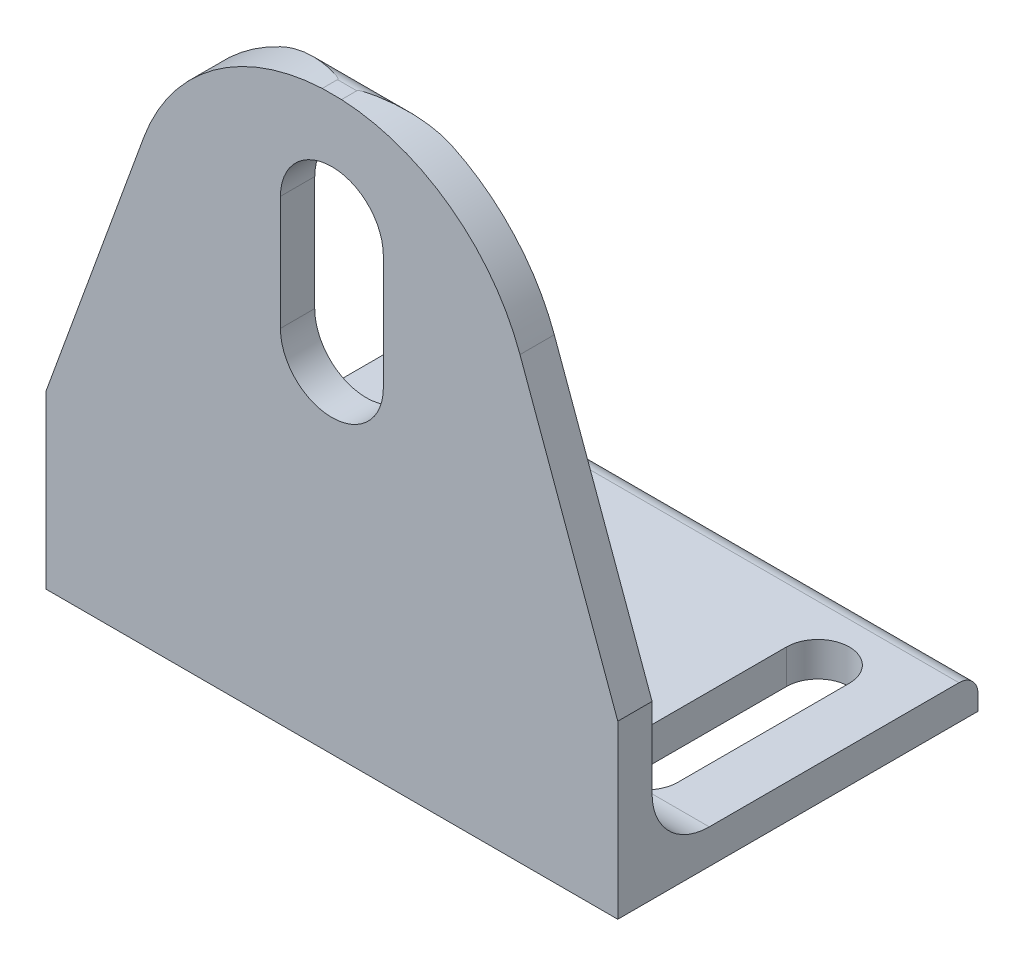
SolidWorks part; units mm, degrees
material "普通碳钢"
ref_plane "Front Plane" through (0, 0, 0) normal (0, 0, 1) x (1, 0, 0)
ref_plane "Top Plane" through (0, 0, 0) normal (0, 1, 0) x (1, 0, 0)
ref_plane "Right Plane" through (0, 0, 0) normal (1, 0, 0) x (0, 0, -1)
sketch3d "3DSketch1"
  line L0 (0, 0, 0) -> (100, 0, 0)
  dimension "D1" = 100
other "Hot-rolled unequal angle gb∕t706-2008 100 X 63 X 6(1)"
ref_plane "Plane1" through (0, 0, 0) normal (1, 0, 0) x (0, 0, -1)
sketch "Sketch1" plane through (0, 0, 0) normal (1, 0, 0) x (0, 0, -1)
  line L0 (0, 0) -> (0, 100)
  line L1 (0, 50) -> (6, 50) construction
  line L2 (6, 96.6667) -> (6, 16)
  line L3 (16, 6) -> (59.6667, 6)
  line L4 (31.5, 6) -> (31.5, 0) construction
  line L5 (63, 0) -> (0, 0)
  line L6 (0, 100) -> (2.6667, 100)
  line L7 (63, 0) -> (63, 2.6667)
  arc A0 (63, 2.6667) -> (59.6667, 6) centre (59.6667, 2.6667) ccw
  arc A1 (2.6667, 100) -> (6, 96.6667) centre (2.6667, 96.6667) cw
  arc A2 (16, 6) -> (6, 16) centre (16, 16) cw
  point P10 (31.5, 0)
  point P14 (0, 50)
  point P15 (6, 50)
  point P16 (31.5, 6)
  point P21 (0, 0)
sketch "Sketch3" plane through (0, 0, 0) normal (0, 0, 1) x (1, 0, 0)
  line L0 (50, 115) -> (50, 0) construction
  line L2 (0, 0) -> (100, 0) construction
  line L3 (50, 80) -> (50, 60) construction
  line L4 (59, 80) -> (59, 60)
  line L5 (41, 80) -> (41, 60)
  line L6 (0, 30) -> (17.101, 76.9846)
  line L7 (0, 100) -> (0, 0) construction
  line L8 (0, 30) -> (0, 0)
  line L9 (0, 0) -> (100, 0)
  line L10 (100, 0) -> (100, 30)
  line L11 (100, 100) -> (100, 0) construction
  line L12 (100, 30) -> (82.899, 76.9846)
  arc A0 (59, 80) -> (41, 80) centre (50, 80) ccw
  arc A1 (41, 60) -> (59, 60) centre (50, 60) ccw
  arc A2 (17.101, 76.9846) -> (82.899, 76.9846) centre (50, 65.0408) cw
  point P8 (50, 70)
  dimension "D6" = 160
  dimension "D8" = 50
  dimension "D9" = 35
  dimension "D1" = 18
  dimension "D2" = 20
  dimension "D3" = 60
  dimension "D4" = 30
  dimension "D5" = 30
  dimension "D7" = 160
extrude "Cut-Extrude1" cut sketch "Sketch3" against normal blind 10 flip side to cut
sketch "Sketch4" plane through (0, 0, 0) normal (0, -1, 0) x (1, 0, 0)
  line L0 (50, 0) -> (50, -67.1057) construction
  line L1 (0, 0) -> (100, 0) construction
  line L3 (15, -20) -> (15, -50) construction
  line L4 (20.5, -20) -> (20.5, -50)
  line L5 (9.5, -20) -> (9.5, -50)
  line L6 (85, -20) -> (85, -50) construction
  line L7 (79.5, -20) -> (79.5, -50)
  line L8 (90.5, -20) -> (90.5, -50)
  line L9 (100, 0) -> (0, 0) construction
  arc A0 (20.5, -20) -> (9.5, -20) centre (15, -20) ccw
  arc A1 (9.5, -50) -> (20.5, -50) centre (15, -50) ccw
  arc A2 (79.5, -20) -> (90.5, -20) centre (85, -20) cw
  arc A3 (90.5, -50) -> (79.5, -50) centre (85, -50) cw
  point P8 (15, -35)
  point P15 (85, -35)
  dimension "D1" = 11
  dimension "D2" = 35
  dimension "D3" = 30
  dimension "D4" = 20
extrude "Cut-Extrude2" cut sketch "Sketch4" against normal blind 15
equation "\"D2@Sketch1\" = \"Radius_1@Sketch1\" / 3"
equation "\"D4@Sketch1\" = \"D1@Sketch1\""
